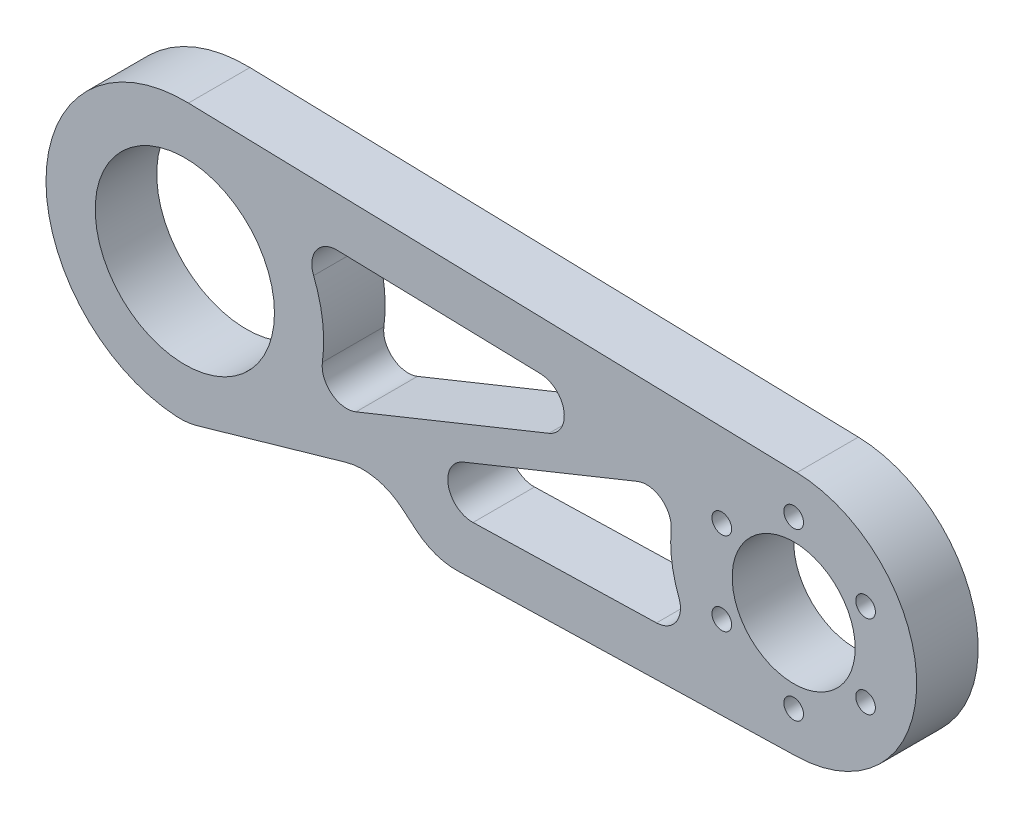
from build123d import *

# Parameters (mm, degrees)
SKETCH_1_R          = 14.575
SKETCH_1_R_2        = 10
EXTRUDE_1_DEPTH     = 10
CUT_EXTRUDE_START   = -10
CUT_EXTRUDE_1_DEPTH = 10
FILLET_1_R          = 4
SKETCH_3_R          = 1.6
CUT_EXTRUDE_2_DEPTH = 10
CUT_EXTRUDE_3_DEPTH = 10
FILLET_2_R          = 10


with BuildPart() as part:
    # 草图1 → 凸台-拉伸1 (new body)
    with BuildSketch(Plane.XY):
        with BuildLine():
            ThreePointArc((0.58717803, 22.567362428), (-22.575, 0), (0.58717803, -22.567362428))
            Line((0.58717803, -22.567362428), (99.52020202, -19.993233602))
            ThreePointArc((99.52020202, -19.993233602), (119, 0), (99.52020202, 19.993233602))
            Line((99.52020202, 19.993233602), (0.58717803, 22.567362428))
        make_face()
        Circle(SKETCH_1_R, mode=Mode.SUBTRACT)
        with Locations((99, 0)):
            Circle(SKETCH_1_R_2, mode=Mode.SUBTRACT)
    extrude(amount=EXTRUDE_1_DEPTH)

    # 草图2 → 切除-拉伸1 (cut)
    with BuildSketch(Plane.XY.offset(10).offset(CUT_EXTRUDE_START)):
        with BuildLine():
            Line((77.045246178, 12.575299839), (17.612754311, 14.121668123))
            ThreePointArc((17.612754311, 14.121668123), (21.298339766, 7.484072969), (22.575, 0))
            ThreePointArc((22.575, 0), (21.923337, -5.384971659), (20.005970563, -10.459051908))
            Line((20.005970563, -10.459051908), (77.045246178, 12.575299839))
        make_face()
        with BuildLine():
            Line((81.037736343, 8.795287621), (24.748948749, -13.935992167))
            Line((24.748948749, -13.935992167), (83.317534331, -12.412101777))
            ThreePointArc((83.317534331, -12.412101777), (79.114570809, -2.137687039), (81.037736343, 8.795287621))
        make_face()
    extrude(amount=CUT_EXTRUDE_1_DEPTH, mode=Mode.SUBTRACT)

    # 圆角1
    fillet_1_edges = [part.edges().sort_by_distance(p)[0] for p in [
        (81.037736343, 8.795287621, 5),
        (83.317534331, -12.412101777, 5),
        (24.748948749, -13.935992167, 5),
        (20.005970563, -10.459051908, 5),
        (17.612754311, 14.121668123, 5),
        (77.045246178, 12.575299839, 5),
    ]]
    fillet(fillet_1_edges, radius=FILLET_1_R)

    # 草图3 → 切除-拉伸2 (cut)
    with BuildSketch(Plane.XY.offset(10)):
        with Locations((99, 13.5)):
            Circle(SKETCH_3_R)
        with Locations((110.691342951, 6.75)):
            Circle(SKETCH_3_R)
        with Locations((110.691342951, -6.75)):
            Circle(SKETCH_3_R)
        with Locations((99, -13.5)):
            Circle(SKETCH_3_R)
        with Locations((87.308657049, -6.75)):
            Circle(SKETCH_3_R)
        with Locations((87.308657049, 6.75)):
            Circle(SKETCH_3_R)
    extrude(amount=-CUT_EXTRUDE_2_DEPTH, mode=Mode.SUBTRACT)

    # 草图4 → 切除-拉伸3 (cut)
    with BuildSketch(Plane.XY.offset(10)):
        Polygon((0.58717803, -22.567362428), (31.302336493, -13.765480202), (40.58717803, -21.526606279), align=None)
    extrude(amount=-CUT_EXTRUDE_3_DEPTH, mode=Mode.SUBTRACT)

    # 圆角2
    fillet_2_edges = [part.edges().sort_by_distance(p)[0] for p in [
        (0.58717803, -22.567362428, 5),
        (40.58717803, -21.526606279, 5),
        (31.302336493, -13.765480202, 5),
    ]]
    fillet(fillet_2_edges, radius=FILLET_2_R)


solid = part.part
